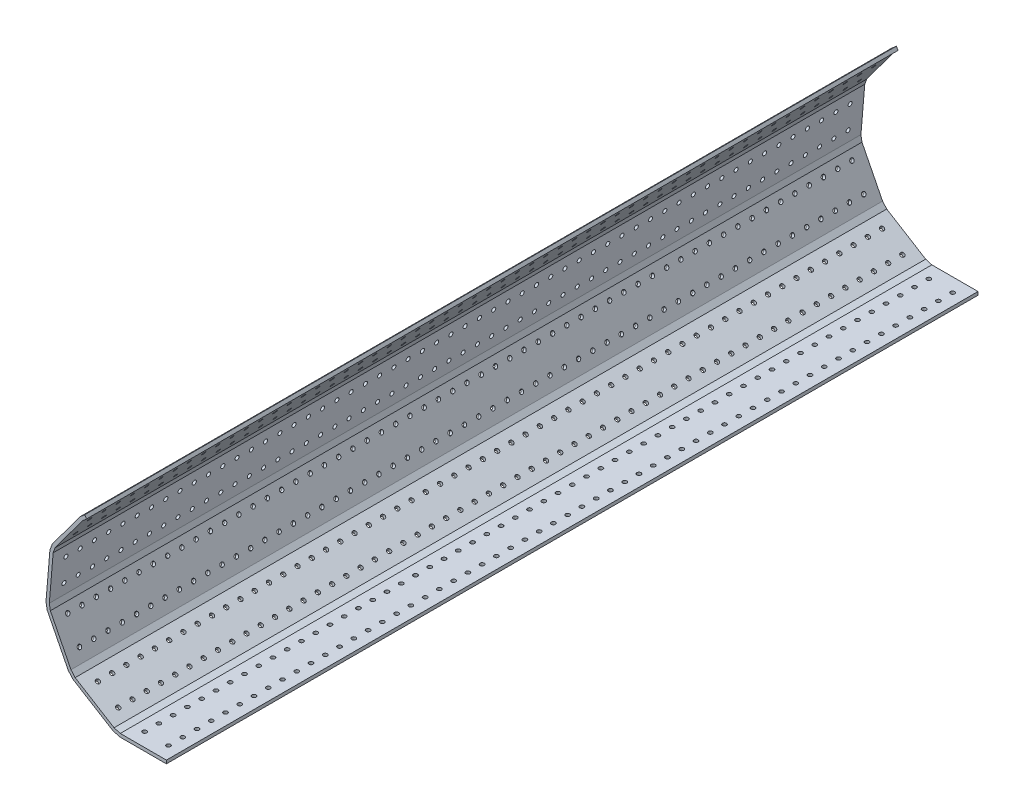
SolidWorks part; units mm, degrees
ref_plane "前视基准面" through (0, 0, 0) normal (0, 0, 1) x (1, 0, 0)
ref_plane "上视基准面" through (0, 0, 0) normal (0, 1, 0) x (1, 0, 0)
ref_plane "右视基准面" through (0, 0, 0) normal (1, 0, 0) x (0, 0, -1)
other "Configuration Table"
sketch "草图5" plane through (0, 0, 0) normal (0, 0, 1) x (1, 0, 0)
  line L12 (10, -352) -> (85, -352)
  line L13 (-85, -352) -> (-10, -352)
  line L14 (-174.7016, -305.0643) -> (-110.8218, -344.3634)
  line L15 (-255.616, -255.2854) -> (-191.7362, -294.5845)
  line L16 (-306.8239, -168.537) -> (-273.0075, -235.4822)
  line L17 (-349.6581, -83.7398) -> (-315.8416, -150.685)
  line L18 (-347.7785, 16.0344) -> (-354.0546, -58.7056)
  line L19 (-339.8288, 110.705) -> (-346.1049, 35.965)
  line L20 (-286.9547, 193.9902) -> (-331.4643, 133.6188)
  line L21 (-230.5758, 270.4605) -> (-275.0855, 210.0892)
  line L22 (-143.2782, 314.1516) -> (-212.8247, 286.053)
  line L23 (-55.1859, 349.7433) -> (-124.7324, 321.6446)
  line L24 (-124.7324, 321.6446) -> (-143.2782, 314.1516)
  line L25 (-212.8247, 286.053) -> (-230.5758, 270.4605)
  line L26 (-275.0855, 210.0892) -> (-286.9547, 193.9902)
  line L27 (-331.4643, 133.6188) -> (-339.8288, 110.705)
  line L28 (-354.0546, -58.7056) -> (-349.6581, -83.7398)
  line L29 (-273.0075, -235.4822) -> (-255.616, -255.2854)
  line L30 (-191.7362, -294.5845) -> (-174.7016, -305.0643)
  line L31 (-110.8218, -344.3634) -> (-85, -352)
  line L32 (-10, -352) -> (10, -352)
  line L34 (-346.1049, 35.965) -> (-347.7785, 16.0344)
  line L35 (-315.8416, -150.685) -> (-306.8239, -168.537)
  line L36 (-138.7829, 303.0254) -> (-206.438, 275.691)
  line L37 (-206.438, 275.691) -> (-221.6847, 262.2984)
  line L38 (-221.6847, 262.2984) -> (-265.4267, 202.9682)
  line L39 (-265.4267, 202.9682) -> (-277.296, 186.8691)
  line L40 (-277.296, 186.8691) -> (-320.7828, 127.8849)
  line L41 (-320.7828, 127.8849) -> (-328.0054, 108.0996)
  line L42 (-328.0054, 108.0996) -> (-334.147, 34.9609)
  line L43 (-334.147, 34.9609) -> (-335.8206, 15.0302)
  line L44 (-335.8206, 15.0302) -> (-341.9666, -58.1608)
  line L45 (-341.9666, -58.1608) -> (-338.1462, -79.9147)
  line L46 (-338.1462, -79.9147) -> (-305.1306, -145.2745)
  line L47 (-305.1306, -145.2745) -> (-296.1129, -163.1265)
  line L48 (-296.1129, -163.1265) -> (-262.9843, -228.7099)
  line L49 (-262.9843, -228.7099) -> (-247.7906, -246.0106)
  line L50 (-247.7906, -246.0106) -> (-185.4483, -284.3638)
  line L51 (-185.4483, -284.3638) -> (-168.4137, -294.8436)
  line L52 (-168.4137, -294.8436) -> (-105.8908, -333.3079)
  line L53 (-105.8908, -333.3079) -> (-83.2627, -340)
  line L54 (-83.2627, -340) -> (-10, -340)
  line L55 (-10, -340) -> (10, -340)
  line L56 (10, -340) -> (85, -340)
  line L58 (-50.6906, 338.617) -> (-120.2371, 310.5184)
  line L59 (-120.2371, 310.5184) -> (-138.7829, 303.0254)
  line L60 (70.3657, -340) -> (-64.1167, 333.1926) construction
  line L61 (85, -352) -> (-55.1859, 349.7433) construction
  line L62 (-55.1859, 349.7433) -> (-50.6906, 338.617)
  line L63 (-64.1167, 333.1926) -> (-120.2371, 310.5184) construction
  line L64 (85, -352) -> (85, -340)
  line L65 (10, -340) -> (70.3657, -340) construction
  dimension "D1" = 12
extrude "凸台-拉伸1" add sketch "草图5" along normal mid plane 2960
sketch "草图6" plane through (0, 0, 1480) normal (0, 0, 1) x (1, 0, 0)
  line L0 (-55.1859, 349.7433) -> (85, -352) construction
  line L1 (14.9071, -1.1284) -> (-1.9629, -1.1284) construction
  circle A3 centre (-1.9629, -1.1284) radius 50
  circle A4 centre (-1.9629, -1.1284) radius 57.5
  dimension "D1" = 16.87
  dimension "D2" = 115
  dimension "D3" = 100
sketch "草图12" plane through (0, -352, 0) normal (0, -1, 0) x (1, 0, 0)
  line L0 (-85, 1480) -> (85, 1480) construction
  line L2 (85, 1480) -> (85, -1480) construction
  line L3 (-1, 1480) -> (-1, 1317.805) construction
  circle A0 centre (42.5, 1429.97) radius 7.5
  circle A1 centre (42.5, 1377.97) radius 7.5
  circle A2 centre (42.5, 1325.97) radius 7.5
  circle A3 centre (42.5, 1273.97) radius 7.5
  circle A4 centre (42.5, 1221.97) radius 7.5
  circle A5 centre (42.5, 1169.97) radius 7.5
  circle A6 centre (42.5, 1117.97) radius 7.5
  circle A7 centre (42.5, 1065.97) radius 7.5
  circle A8 centre (42.5, 1013.97) radius 7.5
  circle A9 centre (42.5, 961.97) radius 7.5
  circle A10 centre (42.5, 909.97) radius 7.5
  circle A11 centre (42.5, 857.97) radius 7.5
  circle A12 centre (42.5, 805.97) radius 7.5
  circle A13 centre (42.5, 753.97) radius 7.5
  circle A14 centre (42.5, 701.97) radius 7.5
  circle A15 centre (42.5, 649.97) radius 7.5
  circle A16 centre (42.5, 597.97) radius 7.5
  circle A17 centre (42.5, 545.97) radius 7.5
  circle A18 centre (42.5, 493.97) radius 7.5
  circle A19 centre (42.5, 441.97) radius 7.5
  circle A20 centre (42.5, 389.97) radius 7.5
  circle A21 centre (42.5, 337.97) radius 7.5
  circle A22 centre (42.5, 285.97) radius 7.5
  circle A23 centre (42.5, 233.97) radius 7.5
  circle A24 centre (42.5, 181.97) radius 7.5
  circle A25 centre (42.5, 129.97) radius 7.5
  circle A26 centre (42.5, 77.97) radius 7.5
  circle A27 centre (42.5, 25.97) radius 7.5
  circle A28 centre (42.5, -26.03) radius 7.5
  circle A29 centre (42.5, -78.03) radius 7.5
  circle A30 centre (42.5, -130.03) radius 7.5
  circle A31 centre (42.5, -182.03) radius 7.5
  circle A32 centre (42.5, -234.03) radius 7.5
  circle A33 centre (42.5, -286.03) radius 7.5
  circle A34 centre (42.5, -338.03) radius 7.5
  circle A35 centre (42.5, -390.03) radius 7.5
  circle A36 centre (42.5, -442.03) radius 7.5
  circle A37 centre (42.5, -494.03) radius 7.5
  circle A38 centre (42.5, -546.03) radius 7.5
  circle A39 centre (42.5, -598.03) radius 7.5
  circle A40 centre (42.5, -650.03) radius 7.5
  circle A41 centre (42.5, -702.03) radius 7.5
  circle A42 centre (42.5, -754.03) radius 7.5
  circle A43 centre (42.5, -806.03) radius 7.5
  circle A44 centre (42.5, -858.03) radius 7.5
  circle A45 centre (42.5, -910.03) radius 7.5
  circle A46 centre (42.5, -962.03) radius 7.5
  circle A47 centre (42.5, -1014.03) radius 7.5
  circle A48 centre (42.5, -1066.03) radius 7.5
  circle A49 centre (42.5, -1118.03) radius 7.5
  circle A50 centre (42.5, -1170.03) radius 7.5
  circle A51 centre (42.5, -1222.03) radius 7.5
  circle A52 centre (-44.5, 1377.97) radius 7.5
  circle A53 centre (-44.5, 1429.97) radius 7.5
  circle A54 centre (-44.5, 1325.97) radius 7.5
  circle A55 centre (-44.5, 1065.97) radius 7.5
  circle A56 centre (-44.5, 1117.97) radius 7.5
  circle A57 centre (-44.5, 1169.97) radius 7.5
  circle A58 centre (-44.5, 1221.97) radius 7.5
  circle A59 centre (-44.5, 1273.97) radius 7.5
  circle A60 centre (-44.5, -1222.03) radius 7.5
  circle A61 centre (-44.5, -1170.03) radius 7.5
  circle A62 centre (-44.5, -1118.03) radius 7.5
  circle A63 centre (-44.5, -1066.03) radius 7.5
  circle A64 centre (-44.5, -1014.03) radius 7.5
  circle A65 centre (-44.5, -962.03) radius 7.5
  circle A66 centre (-44.5, -910.03) radius 7.5
  circle A67 centre (-44.5, -858.03) radius 7.5
  circle A68 centre (-44.5, -806.03) radius 7.5
  circle A69 centre (-44.5, -754.03) radius 7.5
  circle A70 centre (-44.5, -702.03) radius 7.5
  circle A71 centre (-44.5, -650.03) radius 7.5
  circle A72 centre (-44.5, -598.03) radius 7.5
  circle A73 centre (-44.5, -546.03) radius 7.5
  circle A74 centre (-44.5, -494.03) radius 7.5
  circle A75 centre (-44.5, -442.03) radius 7.5
  circle A76 centre (-44.5, -390.03) radius 7.5
  circle A77 centre (-44.5, -338.03) radius 7.5
  circle A78 centre (-44.5, -286.03) radius 7.5
  circle A79 centre (-44.5, -234.03) radius 7.5
  circle A80 centre (-44.5, -182.03) radius 7.5
  circle A81 centre (-44.5, -130.03) radius 7.5
  circle A82 centre (-44.5, -78.03) radius 7.5
  circle A83 centre (-44.5, -26.03) radius 7.5
  circle A84 centre (-44.5, 25.97) radius 7.5
  circle A85 centre (-44.5, 77.97) radius 7.5
  circle A86 centre (-44.5, 129.97) radius 7.5
  circle A87 centre (-44.5, 181.97) radius 7.5
  circle A88 centre (-44.5, 233.97) radius 7.5
  circle A89 centre (-44.5, 285.97) radius 7.5
  circle A90 centre (-44.5, 337.97) radius 7.5
  circle A91 centre (-44.5, 389.97) radius 7.5
  circle A92 centre (-44.5, 441.97) radius 7.5
  circle A93 centre (-44.5, 493.97) radius 7.5
  circle A94 centre (-44.5, 545.97) radius 7.5
  circle A95 centre (-44.5, 597.97) radius 7.5
  circle A96 centre (-44.5, 649.97) radius 7.5
  circle A97 centre (-44.5, 701.97) radius 7.5
  circle A98 centre (-44.5, 753.97) radius 7.5
  circle A99 centre (-44.5, 805.97) radius 7.5
  circle A100 centre (-44.5, 857.97) radius 7.5
  circle A101 centre (-44.5, 909.97) radius 7.5
  circle A102 centre (-44.5, 961.97) radius 7.5
  circle A103 centre (-44.5, 1013.97) radius 7.5
  circle A104 centre (42.5, -1274.03) radius 7.5
  circle A105 centre (42.5, -1326.03) radius 7.5
  circle A106 centre (42.5, -1378.03) radius 7.5
  circle A107 centre (42.5, -1430.03) radius 7.5
  circle A108 centre (-44.5, -1274.03) radius 7.5
  circle A109 centre (-44.5, -1430.03) radius 7.5
  circle A110 centre (-44.5, -1378.03) radius 7.5
  circle A111 centre (-44.5, -1326.03) radius 7.5
  dimension "D2" = 15
  dimension "D1" = 50.03
  dimension "D4" = 52
  dimension "D5" = 42.5
  dimension "D6" = 43.5
  dimension "D3" = 56
extrude "切除-拉伸1" cut sketch "草图12" against normal blind 20
sketch "草图13" plane through (-184.1143, -299.2735, 0) normal (-0.524, -0.8517, 0) x (0.8517, -0.524, 0)
  line L0 (-83.9491, 1480) -> (86.0517, 1480) construction
  line L3 (0.0517, 1480) -> (0.0517, 1394.0275) construction
  line L5 (86.0517, 1480) -> (86.0517, -1480) construction
  circle A0 centre (43.5517, 1429.97) radius 7.5
  circle A1 centre (43.5517, 1377.97) radius 7.5
  circle A2 centre (43.5517, 1325.97) radius 7.5
  circle A3 centre (43.5517, 1273.97) radius 7.5
  circle A4 centre (43.5517, 1221.97) radius 7.5
  circle A5 centre (43.5517, 1169.97) radius 7.5
  circle A6 centre (43.5517, 1117.97) radius 7.5
  circle A7 centre (43.5517, 1065.97) radius 7.5
  circle A8 centre (43.5517, 1013.97) radius 7.5
  circle A9 centre (43.5517, 961.97) radius 7.5
  circle A10 centre (43.5517, 909.97) radius 7.5
  circle A11 centre (43.5517, 857.97) radius 7.5
  circle A12 centre (43.5517, 805.97) radius 7.5
  circle A13 centre (43.5517, 753.97) radius 7.5
  circle A14 centre (43.5517, 701.97) radius 7.5
  circle A15 centre (43.5517, 649.97) radius 7.5
  circle A16 centre (43.5517, 597.97) radius 7.5
  circle A17 centre (43.5517, 545.97) radius 7.5
  circle A18 centre (43.5517, 493.97) radius 7.5
  circle A19 centre (43.5517, 441.97) radius 7.5
  circle A20 centre (43.5517, 389.97) radius 7.5
  circle A21 centre (43.5517, 337.97) radius 7.5
  circle A22 centre (43.5517, 285.97) radius 7.5
  circle A23 centre (43.5517, 233.97) radius 7.5
  circle A24 centre (43.5517, 181.97) radius 7.5
  circle A25 centre (43.5517, 129.97) radius 7.5
  circle A26 centre (43.5517, 77.97) radius 7.5
  circle A27 centre (43.5517, 25.97) radius 7.5
  circle A28 centre (43.5517, -26.03) radius 7.5
  circle A29 centre (43.5517, -78.03) radius 7.5
  circle A30 centre (43.5517, -130.03) radius 7.5
  circle A31 centre (43.5517, -182.03) radius 7.5
  circle A32 centre (43.5517, -234.03) radius 7.5
  circle A33 centre (43.5517, -286.03) radius 7.5
  circle A34 centre (43.5517, -338.03) radius 7.5
  circle A35 centre (43.5517, -390.03) radius 7.5
  circle A36 centre (43.5517, -442.03) radius 7.5
  circle A37 centre (43.5517, -494.03) radius 7.5
  circle A38 centre (43.5517, -546.03) radius 7.5
  circle A39 centre (43.5517, -598.03) radius 7.5
  circle A40 centre (43.5517, -650.03) radius 7.5
  circle A41 centre (43.5517, -702.03) radius 7.5
  circle A42 centre (43.5517, -754.03) radius 7.5
  circle A43 centre (43.5517, -806.03) radius 7.5
  circle A44 centre (43.5517, -858.03) radius 7.5
  circle A45 centre (43.5517, -910.03) radius 7.5
  circle A46 centre (43.5517, -962.03) radius 7.5
  circle A47 centre (43.5517, -1014.03) radius 7.5
  circle A48 centre (43.5517, -1066.03) radius 7.5
  circle A49 centre (43.5517, -1118.03) radius 7.5
  circle A50 centre (43.5517, -1170.03) radius 7.5
  circle A51 centre (43.5517, -1222.03) radius 7.5
  circle A52 centre (43.5517, -1274.03) radius 7.5
  circle A53 centre (43.5517, -1326.03) radius 7.5
  circle A54 centre (43.5517, -1378.03) radius 7.5
  circle A55 centre (43.5517, -1430.03) radius 7.5
  circle A56 centre (-43.4483, 1377.97) radius 7.5
  circle A57 centre (-43.4483, 1429.97) radius 7.5
  circle A58 centre (-43.4483, -1430.03) radius 7.5
  circle A59 centre (-43.4483, -1378.03) radius 7.5
  circle A60 centre (-43.4483, -1326.03) radius 7.5
  circle A61 centre (-43.4483, -1274.03) radius 7.5
  circle A62 centre (-43.4483, -1222.03) radius 7.5
  circle A63 centre (-43.4483, -1170.03) radius 7.5
  circle A64 centre (-43.4483, -1118.03) radius 7.5
  circle A65 centre (-43.4483, -1066.03) radius 7.5
  circle A66 centre (-43.4483, -1014.03) radius 7.5
  circle A67 centre (-43.4483, -962.03) radius 7.5
  circle A68 centre (-43.4483, -910.03) radius 7.5
  circle A69 centre (-43.4483, -858.03) radius 7.5
  circle A70 centre (-43.4483, -806.03) radius 7.5
  circle A71 centre (-43.4483, -754.03) radius 7.5
  circle A72 centre (-43.4483, -702.03) radius 7.5
  circle A73 centre (-43.4483, -650.03) radius 7.5
  circle A74 centre (-43.4483, -598.03) radius 7.5
  circle A75 centre (-43.4483, -546.03) radius 7.5
  circle A76 centre (-43.4483, -494.03) radius 7.5
  circle A77 centre (-43.4483, -442.03) radius 7.5
  circle A78 centre (-43.4483, -390.03) radius 7.5
  circle A79 centre (-43.4483, -338.03) radius 7.5
  circle A80 centre (-43.4483, -286.03) radius 7.5
  circle A81 centre (-43.4483, -234.03) radius 7.5
  circle A82 centre (-43.4483, -182.03) radius 7.5
  circle A83 centre (-43.4483, -130.03) radius 7.5
  circle A84 centre (-43.4483, -78.03) radius 7.5
  circle A85 centre (-43.4483, -26.03) radius 7.5
  circle A86 centre (-43.4483, 25.97) radius 7.5
  circle A87 centre (-43.4483, 77.97) radius 7.5
  circle A88 centre (-43.4483, 129.97) radius 7.5
  circle A89 centre (-43.4483, 181.97) radius 7.5
  circle A90 centre (-43.4483, 233.97) radius 7.5
  circle A91 centre (-43.4483, 285.97) radius 7.5
  circle A92 centre (-43.4483, 337.97) radius 7.5
  circle A93 centre (-43.4483, 389.97) radius 7.5
  circle A94 centre (-43.4483, 441.97) radius 7.5
  circle A95 centre (-43.4483, 493.97) radius 7.5
  circle A96 centre (-43.4483, 545.97) radius 7.5
  circle A97 centre (-43.4483, 597.97) radius 7.5
  circle A98 centre (-43.4483, 649.97) radius 7.5
  circle A99 centre (-43.4483, 701.97) radius 7.5
  circle A100 centre (-43.4483, 753.97) radius 7.5
  circle A101 centre (-43.4483, 805.97) radius 7.5
  circle A102 centre (-43.4483, 857.97) radius 7.5
  circle A103 centre (-43.4483, 909.97) radius 7.5
  circle A104 centre (-43.4483, 961.97) radius 7.5
  circle A105 centre (-43.4483, 1013.97) radius 7.5
  circle A106 centre (-43.4483, 1065.97) radius 7.5
  circle A107 centre (-43.4483, 1117.97) radius 7.5
  circle A108 centre (-43.4483, 1169.97) radius 7.5
  circle A109 centre (-43.4483, 1221.97) radius 7.5
  circle A110 centre (-43.4483, 1273.97) radius 7.5
  circle A111 centre (-43.4483, 1325.97) radius 7.5
  dimension "D2" = 15
  dimension "D1" = 50.03
  dimension "D4" = 52
  dimension "D5" = 42.5
  dimension "D6" = 43.5
  dimension "D3" = 56
extrude "切除-拉伸2" cut sketch "草图13" against normal blind 20
sketch "草图14" plane through (-312.2767, -157.7423, 0) normal (-0.8926, -0.4509, 0) x (0, 0, 1)
  line L0 (-1480, 82.908) -> (-1480, -87.0951) construction
  line L2 (-1480, 3.9049) -> (-1409.6867, 3.9049) construction
  line L4 (1480, -87.0951) -> (-1480, -87.0951) construction
  circle A0 centre (-1429.97, -43.5951) radius 7.5
  circle A1 centre (-1377.97, -43.5951) radius 7.5
  circle A2 centre (-1325.97, -43.5951) radius 7.5
  circle A3 centre (-1273.97, -43.5951) radius 7.5
  circle A4 centre (-1221.97, -43.5951) radius 7.5
  circle A5 centre (-1169.97, -43.5951) radius 7.5
  circle A6 centre (-1117.97, -43.5951) radius 7.5
  circle A7 centre (-1065.97, -43.5951) radius 7.5
  circle A8 centre (-1013.97, -43.5951) radius 7.5
  circle A9 centre (-961.97, -43.5951) radius 7.5
  circle A10 centre (-909.97, -43.5951) radius 7.5
  circle A11 centre (-857.97, -43.5951) radius 7.5
  circle A12 centre (-805.97, -43.5951) radius 7.5
  circle A13 centre (-753.97, -43.5951) radius 7.5
  circle A14 centre (-701.97, -43.5951) radius 7.5
  circle A15 centre (-649.97, -43.5951) radius 7.5
  circle A16 centre (-597.97, -43.5951) radius 7.5
  circle A17 centre (-545.97, -43.5951) radius 7.5
  circle A18 centre (-493.97, -43.5951) radius 7.5
  circle A19 centre (-441.97, -43.5951) radius 7.5
  circle A20 centre (-389.97, -43.5951) radius 7.5
  circle A21 centre (-337.97, -43.5951) radius 7.5
  circle A22 centre (-285.97, -43.5951) radius 7.5
  circle A23 centre (-233.97, -43.5951) radius 7.5
  circle A24 centre (-181.97, -43.5951) radius 7.5
  circle A25 centre (-129.97, -43.5951) radius 7.5
  circle A26 centre (-77.97, -43.5951) radius 7.5
  circle A27 centre (-25.97, -43.5951) radius 7.5
  circle A28 centre (26.03, -43.5951) radius 7.5
  circle A29 centre (78.03, -43.5951) radius 7.5
  circle A30 centre (130.03, -43.5951) radius 7.5
  circle A31 centre (182.03, -43.5951) radius 7.5
  circle A32 centre (234.03, -43.5951) radius 7.5
  circle A33 centre (286.03, -43.5951) radius 7.5
  circle A34 centre (338.03, -43.5951) radius 7.5
  circle A35 centre (390.03, -43.5951) radius 7.5
  circle A36 centre (442.03, -43.5951) radius 7.5
  circle A37 centre (494.03, -43.5951) radius 7.5
  circle A38 centre (546.03, -43.5951) radius 7.5
  circle A39 centre (598.03, -43.5951) radius 7.5
  circle A40 centre (650.03, -43.5951) radius 7.5
  circle A41 centre (702.03, -43.5951) radius 7.5
  circle A42 centre (754.03, -43.5951) radius 7.5
  circle A43 centre (806.03, -43.5951) radius 7.5
  circle A44 centre (858.03, -43.5951) radius 7.5
  circle A45 centre (910.03, -43.5951) radius 7.5
  circle A46 centre (962.03, -43.5951) radius 7.5
  circle A47 centre (1014.03, -43.5951) radius 7.5
  circle A48 centre (1066.03, -43.5951) radius 7.5
  circle A49 centre (1118.03, -43.5951) radius 7.5
  circle A50 centre (1170.03, -43.5951) radius 7.5
  circle A51 centre (1222.03, -43.5951) radius 7.5
  circle A52 centre (1274.03, -43.5951) radius 7.5
  circle A53 centre (1326.03, -43.5951) radius 7.5
  circle A54 centre (1378.03, -43.5951) radius 7.5
  circle A55 centre (1430.03, -43.5951) radius 7.5
  circle A56 centre (1430.03, 51.4049) radius 7.5
  circle A57 centre (1378.03, 51.4049) radius 7.5
  circle A58 centre (1326.03, 51.4049) radius 7.5
  circle A59 centre (1274.03, 51.4049) radius 7.5
  circle A60 centre (1222.03, 51.4049) radius 7.5
  circle A61 centre (1170.03, 51.4049) radius 7.5
  circle A62 centre (1118.03, 51.4049) radius 7.5
  circle A63 centre (1066.03, 51.4049) radius 7.5
  circle A64 centre (1014.03, 51.4049) radius 7.5
  circle A65 centre (962.03, 51.4049) radius 7.5
  circle A66 centre (910.03, 51.4049) radius 7.5
  circle A67 centre (858.03, 51.4049) radius 7.5
  circle A68 centre (806.03, 51.4049) radius 7.5
  circle A69 centre (754.03, 51.4049) radius 7.5
  circle A70 centre (702.03, 51.4049) radius 7.5
  circle A71 centre (650.03, 51.4049) radius 7.5
  circle A72 centre (598.03, 51.4049) radius 7.5
  circle A73 centre (546.03, 51.4049) radius 7.5
  circle A74 centre (494.03, 51.4049) radius 7.5
  circle A75 centre (442.03, 51.4049) radius 7.5
  circle A76 centre (390.03, 51.4049) radius 7.5
  circle A77 centre (338.03, 51.4049) radius 7.5
  circle A78 centre (286.03, 51.4049) radius 7.5
  circle A79 centre (234.03, 51.4049) radius 7.5
  circle A80 centre (182.03, 51.4049) radius 7.5
  circle A81 centre (130.03, 51.4049) radius 7.5
  circle A82 centre (78.03, 51.4049) radius 7.5
  circle A83 centre (26.03, 51.4049) radius 7.5
  circle A84 centre (-25.97, 51.4049) radius 7.5
  circle A85 centre (-77.97, 51.4049) radius 7.5
  circle A86 centre (-129.97, 51.4049) radius 7.5
  circle A87 centre (-181.97, 51.4049) radius 7.5
  circle A88 centre (-233.97, 51.4049) radius 7.5
  circle A89 centre (-285.97, 51.4049) radius 7.5
  circle A90 centre (-337.97, 51.4049) radius 7.5
  circle A91 centre (-389.97, 51.4049) radius 7.5
  circle A92 centre (-441.97, 51.4049) radius 7.5
  circle A93 centre (-493.97, 51.4049) radius 7.5
  circle A94 centre (-545.97, 51.4049) radius 7.5
  circle A95 centre (-597.97, 51.4049) radius 7.5
  circle A96 centre (-649.97, 51.4049) radius 7.5
  circle A97 centre (-701.97, 51.4049) radius 7.5
  circle A98 centre (-753.97, 51.4049) radius 7.5
  circle A99 centre (-805.97, 51.4049) radius 7.5
  circle A100 centre (-857.97, 51.4049) radius 7.5
  circle A101 centre (-909.97, 51.4049) radius 7.5
  circle A102 centre (-961.97, 51.4049) radius 7.5
  circle A103 centre (-1013.97, 51.4049) radius 7.5
  circle A104 centre (-1065.97, 51.4049) radius 7.5
  circle A105 centre (-1117.97, 51.4049) radius 7.5
  circle A106 centre (-1169.97, 51.4049) radius 7.5
  circle A107 centre (-1221.97, 51.4049) radius 7.5
  circle A108 centre (-1273.97, 51.4049) radius 7.5
  circle A109 centre (-1325.97, 51.4049) radius 7.5
  circle A110 centre (-1377.97, 51.4049) radius 7.5
  circle A111 centre (-1429.97, 51.4049) radius 7.5
  dimension "D1" = 15
  dimension "D2" = 50.03
  dimension "D4" = 52
  dimension "D5" = 43.5
  dimension "D6" = 95
  dimension "D3" = 56
extrude "切除-拉伸3" cut sketch "草图14" against normal blind 20
sketch3d "3D草图1" [suppressed]
  line L0 (-351.8563, -71.2227, 1480) -> (-351.8563, -71.2227, -1480)
  line L1 (-354.0546, -58.7056, 1480) -> (-349.6581, -83.7398, 1480) construction
  line L2 (-354.0546, -58.7056, -1480) -> (-349.6581, -83.7398, -1480) construction
sketch3d "3D草图3" [suppressed]
  line L0 (-340.0564, -69.0378, 1480) -> (-340.0564, -69.0378, -1480)
  line L3 (-338.1462, -79.9147, 1480) -> (-341.9666, -58.1608, 1480) construction
  line L4 (-338.1462, -79.9147, -1480) -> (-341.9666, -58.1608, -1480) construction
sketch3d "3D草图4" [suppressed]
  line L0 (-351.8563, -71.2227, 1480) -> (-340.0564, -69.0378, 1480)
  line L1 (-354.0546, -58.7056, 1480) -> (-349.6581, -83.7398, 1480) construction
  line L2 (-338.1462, -79.9147, 1480) -> (-341.9666, -58.1608, 1480) construction
sketch "草图15" plane through (-346.6804, 29.1116, 0) normal (-0.9965, 0.0837, 0) x (0, 0, 1)
  line L0 (-1480, 81.8806) -> (-1480, -88.1263) construction
  line L1 (1480, -88.1263) -> (-1480, -88.1263) construction
  line L2 (-1480, -2.1263) -> (-1352.9164, -2.1263) construction
  circle A0 centre (-1429.97, -45.6263) radius 7.5
  circle A1 centre (-1377.97, -45.6263) radius 7.5
  circle A2 centre (-1325.97, -45.6263) radius 7.5
  circle A3 centre (-1273.97, -45.6263) radius 7.5
  circle A4 centre (-1221.97, -45.6263) radius 7.5
  circle A5 centre (-1169.97, -45.6263) radius 7.5
  circle A6 centre (-1117.97, -45.6263) radius 7.5
  circle A7 centre (-1065.97, -45.6263) radius 7.5
  circle A8 centre (-1013.97, -45.6263) radius 7.5
  circle A9 centre (-961.97, -45.6263) radius 7.5
  circle A10 centre (-909.97, -45.6263) radius 7.5
  circle A11 centre (-857.97, -45.6263) radius 7.5
  circle A12 centre (-805.97, -45.6263) radius 7.5
  circle A13 centre (-753.97, -45.6263) radius 7.5
  circle A14 centre (-701.97, -45.6263) radius 7.5
  circle A15 centre (-649.97, -45.6263) radius 7.5
  circle A16 centre (-597.97, -45.6263) radius 7.5
  circle A17 centre (-545.97, -45.6263) radius 7.5
  circle A18 centre (-493.97, -45.6263) radius 7.5
  circle A19 centre (-441.97, -45.6263) radius 7.5
  circle A20 centre (-389.97, -45.6263) radius 7.5
  circle A21 centre (-337.97, -45.6263) radius 7.5
  circle A22 centre (-285.97, -45.6263) radius 7.5
  circle A23 centre (-233.97, -45.6263) radius 7.5
  circle A24 centre (-181.97, -45.6263) radius 7.5
  circle A25 centre (-129.97, -45.6263) radius 7.5
  circle A26 centre (-77.97, -45.6263) radius 7.5
  circle A27 centre (-25.97, -45.6263) radius 7.5
  circle A28 centre (26.03, -45.6263) radius 7.5
  circle A29 centre (78.03, -45.6263) radius 7.5
  circle A30 centre (130.03, -45.6263) radius 7.5
  circle A31 centre (182.03, -45.6263) radius 7.5
  circle A32 centre (234.03, -45.6263) radius 7.5
  circle A33 centre (286.03, -45.6263) radius 7.5
  circle A34 centre (338.03, -45.6263) radius 7.5
  circle A35 centre (390.03, -45.6263) radius 7.5
  circle A36 centre (442.03, -45.6263) radius 7.5
  circle A37 centre (494.03, -45.6263) radius 7.5
  circle A38 centre (546.03, -45.6263) radius 7.5
  circle A39 centre (598.03, -45.6263) radius 7.5
  circle A40 centre (650.03, -45.6263) radius 7.5
  circle A41 centre (702.03, -45.6263) radius 7.5
  circle A42 centre (754.03, -45.6263) radius 7.5
  circle A43 centre (806.03, -45.6263) radius 7.5
  circle A44 centre (858.03, -45.6263) radius 7.5
  circle A45 centre (910.03, -45.6263) radius 7.5
  circle A46 centre (962.03, -45.6263) radius 7.5
  circle A47 centre (1014.03, -45.6263) radius 7.5
  circle A48 centre (1066.03, -45.6263) radius 7.5
  circle A49 centre (1118.03, -45.6263) radius 7.5
  circle A50 centre (1170.03, -45.6263) radius 7.5
  circle A51 centre (1222.03, -45.6263) radius 7.5
  circle A52 centre (1274.03, -45.6263) radius 7.5
  circle A53 centre (1326.03, -45.6263) radius 7.5
  circle A54 centre (1378.03, -45.6263) radius 7.5
  circle A55 centre (1430.03, -45.6263) radius 7.5
  circle A56 centre (1430.03, 41.3737) radius 7.5
  circle A57 centre (1378.03, 41.3737) radius 7.5
  circle A58 centre (1326.03, 41.3737) radius 7.5
  circle A59 centre (1274.03, 41.3737) radius 7.5
  circle A60 centre (1222.03, 41.3737) radius 7.5
  circle A61 centre (1170.03, 41.3737) radius 7.5
  circle A62 centre (1118.03, 41.3737) radius 7.5
  circle A63 centre (1066.03, 41.3737) radius 7.5
  circle A64 centre (1014.03, 41.3737) radius 7.5
  circle A65 centre (962.03, 41.3737) radius 7.5
  circle A66 centre (910.03, 41.3737) radius 7.5
  circle A67 centre (858.03, 41.3737) radius 7.5
  circle A68 centre (806.03, 41.3737) radius 7.5
  circle A69 centre (754.03, 41.3737) radius 7.5
  circle A70 centre (702.03, 41.3737) radius 7.5
  circle A71 centre (650.03, 41.3737) radius 7.5
  circle A72 centre (598.03, 41.3737) radius 7.5
  circle A73 centre (546.03, 41.3737) radius 7.5
  circle A74 centre (494.03, 41.3737) radius 7.5
  circle A75 centre (442.03, 41.3737) radius 7.5
  circle A76 centre (390.03, 41.3737) radius 7.5
  circle A77 centre (338.03, 41.3737) radius 7.5
  circle A78 centre (286.03, 41.3737) radius 7.5
  circle A79 centre (234.03, 41.3737) radius 7.5
  circle A80 centre (182.03, 41.3737) radius 7.5
  circle A81 centre (130.03, 41.3737) radius 7.5
  circle A82 centre (78.03, 41.3737) radius 7.5
  circle A83 centre (26.03, 41.3737) radius 7.5
  circle A84 centre (-25.97, 41.3737) radius 7.5
  circle A85 centre (-77.97, 41.3737) radius 7.5
  circle A86 centre (-129.97, 41.3737) radius 7.5
  circle A87 centre (-181.97, 41.3737) radius 7.5
  circle A88 centre (-233.97, 41.3737) radius 7.5
  circle A89 centre (-285.97, 41.3737) radius 7.5
  circle A90 centre (-337.97, 41.3737) radius 7.5
  circle A91 centre (-389.97, 41.3737) radius 7.5
  circle A92 centre (-441.97, 41.3737) radius 7.5
  circle A93 centre (-493.97, 41.3737) radius 7.5
  circle A94 centre (-545.97, 41.3737) radius 7.5
  circle A95 centre (-597.97, 41.3737) radius 7.5
  circle A96 centre (-649.97, 41.3737) radius 7.5
  circle A97 centre (-701.97, 41.3737) radius 7.5
  circle A98 centre (-753.97, 41.3737) radius 7.5
  circle A99 centre (-805.97, 41.3737) radius 7.5
  circle A100 centre (-857.97, 41.3737) radius 7.5
  circle A101 centre (-909.97, 41.3737) radius 7.5
  circle A102 centre (-961.97, 41.3737) radius 7.5
  circle A103 centre (-1013.97, 41.3737) radius 7.5
  circle A104 centre (-1065.97, 41.3737) radius 7.5
  circle A105 centre (-1117.97, 41.3737) radius 7.5
  circle A106 centre (-1169.97, 41.3737) radius 7.5
  circle A107 centre (-1221.97, 41.3737) radius 7.5
  circle A108 centre (-1273.97, 41.3737) radius 7.5
  circle A109 centre (-1325.97, 41.3737) radius 7.5
  circle A110 centre (-1377.97, 41.3737) radius 7.5
  circle A111 centre (-1429.97, 41.3737) radius 7.5
  dimension "D1" = 15
  dimension "D2" = 50.03
  dimension "D4" = 52
  dimension "D5" = 42.5
  dimension "D6" = 87
  dimension "D3" = 56
sketch "草图16" plane through (-278.562, 205.3736, 0) normal (-0.8049, 0.5934, 0) x (0, 0, 1)
  line L0 (-1480, 80.8639) -> (-1480, -89.1482) construction
  line L1 (1480, -89.1482) -> (-1480, -89.1482) construction
  line L2 (-1480, -3.1482) -> (-1338.0926, -3.1482) construction
  circle A0 centre (-1429.97, -46.6482) radius 7.5
  circle A1 centre (-1377.97, -46.6482) radius 7.5
  circle A2 centre (-1325.97, -46.6482) radius 7.5
  circle A3 centre (-1273.97, -46.6482) radius 7.5
  circle A4 centre (-1221.97, -46.6482) radius 7.5
  circle A5 centre (-1169.97, -46.6482) radius 7.5
  circle A6 centre (-1117.97, -46.6482) radius 7.5
  circle A7 centre (-1065.97, -46.6482) radius 7.5
  circle A8 centre (-1013.97, -46.6482) radius 7.5
  circle A9 centre (-961.97, -46.6482) radius 7.5
  circle A10 centre (-909.97, -46.6482) radius 7.5
  circle A11 centre (-857.97, -46.6482) radius 7.5
  circle A12 centre (-805.97, -46.6482) radius 7.5
  circle A13 centre (-753.97, -46.6482) radius 7.5
  circle A14 centre (-701.97, -46.6482) radius 7.5
  circle A15 centre (-649.97, -46.6482) radius 7.5
  circle A16 centre (-597.97, -46.6482) radius 7.5
  circle A17 centre (-545.97, -46.6482) radius 7.5
  circle A18 centre (-493.97, -46.6482) radius 7.5
  circle A19 centre (-441.97, -46.6482) radius 7.5
  circle A20 centre (-389.97, -46.6482) radius 7.5
  circle A21 centre (-337.97, -46.6482) radius 7.5
  circle A22 centre (-285.97, -46.6482) radius 7.5
  circle A23 centre (-233.97, -46.6482) radius 7.5
  circle A24 centre (-181.97, -46.6482) radius 7.5
  circle A25 centre (-129.97, -46.6482) radius 7.5
  circle A26 centre (-77.97, -46.6482) radius 7.5
  circle A27 centre (-25.97, -46.6482) radius 7.5
  circle A28 centre (26.03, -46.6482) radius 7.5
  circle A29 centre (78.03, -46.6482) radius 7.5
  circle A30 centre (130.03, -46.6482) radius 7.5
  circle A31 centre (182.03, -46.6482) radius 7.5
  circle A32 centre (234.03, -46.6482) radius 7.5
  circle A33 centre (286.03, -46.6482) radius 7.5
  circle A34 centre (338.03, -46.6482) radius 7.5
  circle A35 centre (390.03, -46.6482) radius 7.5
  circle A36 centre (442.03, -46.6482) radius 7.5
  circle A37 centre (494.03, -46.6482) radius 7.5
  circle A38 centre (546.03, -46.6482) radius 7.5
  circle A39 centre (598.03, -46.6482) radius 7.5
  circle A40 centre (650.03, -46.6482) radius 7.5
  circle A41 centre (702.03, -46.6482) radius 7.5
  circle A42 centre (754.03, -46.6482) radius 7.5
  circle A43 centre (806.03, -46.6482) radius 7.5
  circle A44 centre (858.03, -46.6482) radius 7.5
  circle A45 centre (910.03, -46.6482) radius 7.5
  circle A46 centre (962.03, -46.6482) radius 7.5
  circle A47 centre (1014.03, -46.6482) radius 7.5
  circle A48 centre (1066.03, -46.6482) radius 7.5
  circle A49 centre (1118.03, -46.6482) radius 7.5
  circle A50 centre (1170.03, -46.6482) radius 7.5
  circle A51 centre (1222.03, -46.6482) radius 7.5
  circle A52 centre (1274.03, -46.6482) radius 7.5
  circle A53 centre (1326.03, -46.6482) radius 7.5
  circle A54 centre (1378.03, -46.6482) radius 7.5
  circle A55 centre (1430.03, -46.6482) radius 7.5
  circle A56 centre (1430.03, 40.3518) radius 7.5
  circle A57 centre (1378.03, 40.3518) radius 7.5
  circle A58 centre (1326.03, 40.3518) radius 7.5
  circle A59 centre (1274.03, 40.3518) radius 7.5
  circle A60 centre (1222.03, 40.3518) radius 7.5
  circle A61 centre (1170.03, 40.3518) radius 7.5
  circle A62 centre (1118.03, 40.3518) radius 7.5
  circle A63 centre (1066.03, 40.3518) radius 7.5
  circle A64 centre (1014.03, 40.3518) radius 7.5
  circle A65 centre (962.03, 40.3518) radius 7.5
  circle A66 centre (910.03, 40.3518) radius 7.5
  circle A67 centre (858.03, 40.3518) radius 7.5
  circle A68 centre (806.03, 40.3518) radius 7.5
  circle A69 centre (754.03, 40.3518) radius 7.5
  circle A70 centre (702.03, 40.3518) radius 7.5
  circle A71 centre (650.03, 40.3518) radius 7.5
  circle A72 centre (598.03, 40.3518) radius 7.5
  circle A73 centre (546.03, 40.3518) radius 7.5
  circle A74 centre (494.03, 40.3518) radius 7.5
  circle A75 centre (442.03, 40.3518) radius 7.5
  circle A76 centre (390.03, 40.3518) radius 7.5
  circle A77 centre (338.03, 40.3518) radius 7.5
  circle A78 centre (286.03, 40.3518) radius 7.5
  circle A79 centre (234.03, 40.3518) radius 7.5
  circle A80 centre (182.03, 40.3518) radius 7.5
  circle A81 centre (130.03, 40.3518) radius 7.5
  circle A82 centre (78.03, 40.3518) radius 7.5
  circle A83 centre (26.03, 40.3518) radius 7.5
  circle A84 centre (-25.97, 40.3518) radius 7.5
  circle A85 centre (-77.97, 40.3518) radius 7.5
  circle A86 centre (-129.97, 40.3518) radius 7.5
  circle A87 centre (-181.97, 40.3518) radius 7.5
  circle A88 centre (-233.97, 40.3518) radius 7.5
  circle A89 centre (-285.97, 40.3518) radius 7.5
  circle A90 centre (-337.97, 40.3518) radius 7.5
  circle A91 centre (-389.97, 40.3518) radius 7.5
  circle A92 centre (-441.97, 40.3518) radius 7.5
  circle A93 centre (-493.97, 40.3518) radius 7.5
  circle A94 centre (-545.97, 40.3518) radius 7.5
  circle A95 centre (-597.97, 40.3518) radius 7.5
  circle A96 centre (-649.97, 40.3518) radius 7.5
  circle A97 centre (-701.97, 40.3518) radius 7.5
  circle A98 centre (-753.97, 40.3518) radius 7.5
  circle A99 centre (-805.97, 40.3518) radius 7.5
  circle A100 centre (-857.97, 40.3518) radius 7.5
  circle A101 centre (-909.97, 40.3518) radius 7.5
  circle A102 centre (-961.97, 40.3518) radius 7.5
  circle A103 centre (-1013.97, 40.3518) radius 7.5
  circle A104 centre (-1065.97, 40.3518) radius 7.5
  circle A105 centre (-1117.97, 40.3518) radius 7.5
  circle A106 centre (-1169.97, 40.3518) radius 7.5
  circle A107 centre (-1221.97, 40.3518) radius 7.5
  circle A108 centre (-1273.97, 40.3518) radius 7.5
  circle A109 centre (-1325.97, 40.3518) radius 7.5
  circle A110 centre (-1377.97, 40.3518) radius 7.5
  circle A111 centre (-1429.97, 40.3518) radius 7.5
  dimension "D1" = 15
  dimension "D4" = 52
  dimension "D2" = 50.03
  dimension "D5" = 42.5
  dimension "D6" = 87
  dimension "D3" = 56
sketch "草图17" plane through (-129.2203, 319.8314, 0) normal (-0.3746, 0.9272, 0) x (0.9272, 0.3746, 0)
  line L0 (79.8487, 1480) -> (-90.1703, 1480) construction
  line L2 (-0.1703, 1480) -> (-0.1703, 1377.97) construction
  line L3 (-90.1703, -1480) -> (-90.1703, 1480) construction
  circle A0 centre (47.3297, 1429.97) radius 15
  circle A1 centre (47.3297, 1377.97) radius 15
  circle A2 centre (47.3297, 1325.97) radius 15
  circle A3 centre (47.3297, 1273.97) radius 15
  circle A4 centre (47.3297, 1221.97) radius 15
  circle A5 centre (47.3297, 1169.97) radius 15
  circle A6 centre (47.3297, 1117.97) radius 15
  circle A7 centre (47.3297, 1065.97) radius 15
  circle A8 centre (47.3297, 1013.97) radius 15
  circle A9 centre (47.3297, 961.97) radius 15
  circle A10 centre (47.3297, 909.97) radius 15
  circle A11 centre (47.3297, 857.97) radius 15
  circle A12 centre (47.3297, 805.97) radius 15
  circle A13 centre (47.3297, 753.97) radius 15
  circle A14 centre (47.3297, 701.97) radius 15
  circle A15 centre (47.3297, 649.97) radius 15
  circle A16 centre (47.3297, 597.97) radius 15
  circle A17 centre (47.3297, 545.97) radius 15
  circle A18 centre (47.3297, 493.97) radius 15
  circle A19 centre (47.3297, 441.97) radius 15
  circle A20 centre (47.3297, 389.97) radius 15
  circle A21 centre (47.3297, 337.97) radius 15
  circle A22 centre (47.3297, 285.97) radius 15
  circle A23 centre (47.3297, 233.97) radius 15
  circle A24 centre (47.3297, 181.97) radius 15
  circle A25 centre (47.3297, 129.97) radius 15
  circle A26 centre (47.3297, 77.97) radius 15
  circle A27 centre (47.3297, 25.97) radius 15
  circle A28 centre (47.3297, -26.03) radius 15
  circle A29 centre (47.3297, -78.03) radius 15
  circle A30 centre (47.3297, -130.03) radius 15
  circle A31 centre (47.3297, -182.03) radius 15
  circle A32 centre (47.3297, -234.03) radius 15
  circle A33 centre (47.3297, -286.03) radius 15
  circle A34 centre (47.3297, -338.03) radius 15
  circle A35 centre (47.3297, -390.03) radius 15
  circle A36 centre (47.3297, -442.03) radius 15
  circle A37 centre (47.3297, -494.03) radius 15
  circle A38 centre (47.3297, -546.03) radius 15
  circle A39 centre (47.3297, -598.03) radius 15
  circle A40 centre (47.3297, -650.03) radius 15
  circle A41 centre (47.3297, -702.03) radius 15
  circle A42 centre (47.3297, -754.03) radius 15
  circle A43 centre (47.3297, -806.03) radius 15
  circle A44 centre (47.3297, -858.03) radius 15
  circle A45 centre (47.3297, -910.03) radius 15
  circle A46 centre (47.3297, -962.03) radius 15
  circle A47 centre (47.3297, -1014.03) radius 15
  circle A48 centre (47.3297, -1066.03) radius 15
  circle A49 centre (47.3297, -1118.03) radius 15
  circle A50 centre (47.3297, -1170.03) radius 15
  circle A51 centre (47.3297, -1222.03) radius 15
  circle A52 centre (47.3297, -1274.03) radius 15
  circle A53 centre (47.3297, -1326.03) radius 15
  circle A54 centre (47.3297, -1378.03) radius 15
  circle A55 centre (47.3297, -1430.03) radius 15
  circle A56 centre (-47.6703, -1430.03) radius 15
  circle A57 centre (-47.6703, -1378.03) radius 15
  circle A58 centre (-47.6703, -1326.03) radius 15
  circle A59 centre (-47.6703, -1274.03) radius 15
  circle A60 centre (-47.6703, -1222.03) radius 15
  circle A61 centre (-47.6703, -1170.03) radius 15
  circle A62 centre (-47.6703, -1118.03) radius 15
  circle A63 centre (-47.6703, -1066.03) radius 15
  circle A64 centre (-47.6703, -1014.03) radius 15
  circle A65 centre (-47.6703, -962.03) radius 15
  circle A66 centre (-47.6703, -910.03) radius 15
  circle A67 centre (-47.6703, -858.03) radius 15
  circle A68 centre (-47.6703, -806.03) radius 15
  circle A69 centre (-47.6703, -754.03) radius 15
  circle A70 centre (-47.6703, -702.03) radius 15
  circle A71 centre (-47.6703, -650.03) radius 15
  circle A72 centre (-47.6703, -598.03) radius 15
  circle A73 centre (-47.6703, -546.03) radius 15
  circle A74 centre (-47.6703, -494.03) radius 15
  circle A75 centre (-47.6703, -442.03) radius 15
  circle A76 centre (-47.6703, -390.03) radius 15
  circle A77 centre (-47.6703, -338.03) radius 15
  circle A78 centre (-47.6703, -286.03) radius 15
  circle A79 centre (-47.6703, -234.03) radius 15
  circle A80 centre (-47.6703, -182.03) radius 15
  circle A81 centre (-47.6703, -130.03) radius 15
  circle A82 centre (-47.6703, -78.03) radius 15
  circle A83 centre (-47.6703, -26.03) radius 15
  circle A84 centre (-47.6703, 25.97) radius 15
  circle A85 centre (-47.6703, 77.97) radius 15
  circle A86 centre (-47.6703, 129.97) radius 15
  circle A87 centre (-47.6703, 181.97) radius 15
  circle A88 centre (-47.6703, 233.97) radius 15
  circle A89 centre (-47.6703, 285.97) radius 15
  circle A90 centre (-47.6703, 337.97) radius 15
  circle A91 centre (-47.6703, 389.97) radius 15
  circle A92 centre (-47.6703, 441.97) radius 15
  circle A93 centre (-47.6703, 493.97) radius 15
  circle A94 centre (-47.6703, 545.97) radius 15
  circle A95 centre (-47.6703, 597.97) radius 15
  circle A96 centre (-47.6703, 649.97) radius 15
  circle A97 centre (-47.6703, 701.97) radius 15
  circle A98 centre (-47.6703, 753.97) radius 15
  circle A99 centre (-47.6703, 805.97) radius 15
  circle A100 centre (-47.6703, 857.97) radius 15
  circle A101 centre (-47.6703, 909.97) radius 15
  circle A102 centre (-47.6703, 961.97) radius 15
  circle A103 centre (-47.6703, 1013.97) radius 15
  circle A104 centre (-47.6703, 1065.97) radius 15
  circle A105 centre (-47.6703, 1117.97) radius 15
  circle A106 centre (-47.6703, 1169.97) radius 15
  circle A107 centre (-47.6703, 1221.97) radius 15
  circle A108 centre (-47.6703, 1273.97) radius 15
  circle A109 centre (-47.6703, 1325.97) radius 15
  circle A110 centre (-47.6703, 1377.97) radius 15
  circle A111 centre (-47.6703, 1429.97) radius 15
  dimension "D2" = 30
  dimension "D1" = 50.03
  dimension "D4" = 52
  dimension "D5" = 42.5
  dimension "D6" = 95
  dimension "D3" = 56
extrude "切除-拉伸5" cut sketch "草图16" against normal blind 20
extrude "切除-拉伸6" cut sketch "草图15" against normal blind 20
extrude "切除-拉伸7" cut sketch "草图17" against normal blind 20
sketch "草图18" plane through (0, 0, 1480) normal (0, 0, 1) x (1, 0, 0)
  line L0 (-206.438, 275.691) -> (-50.6906, 338.617) construction
  line L1 (-55.1859, 349.7433) -> (-212.8247, 286.053) construction
  line L2 (-206.438, 275.691) -> (-50.6906, 338.617)
  line L3 (-55.1859, 349.7433) -> (-212.8247, 286.053)
  line L4 (-212.8247, 286.053) -> (-206.438, 275.691)
  line L5 (-55.1859, 349.7433) -> (-50.6906, 338.617)
extrude "切除-拉伸8" cut sketch "草图18" against normal through all
